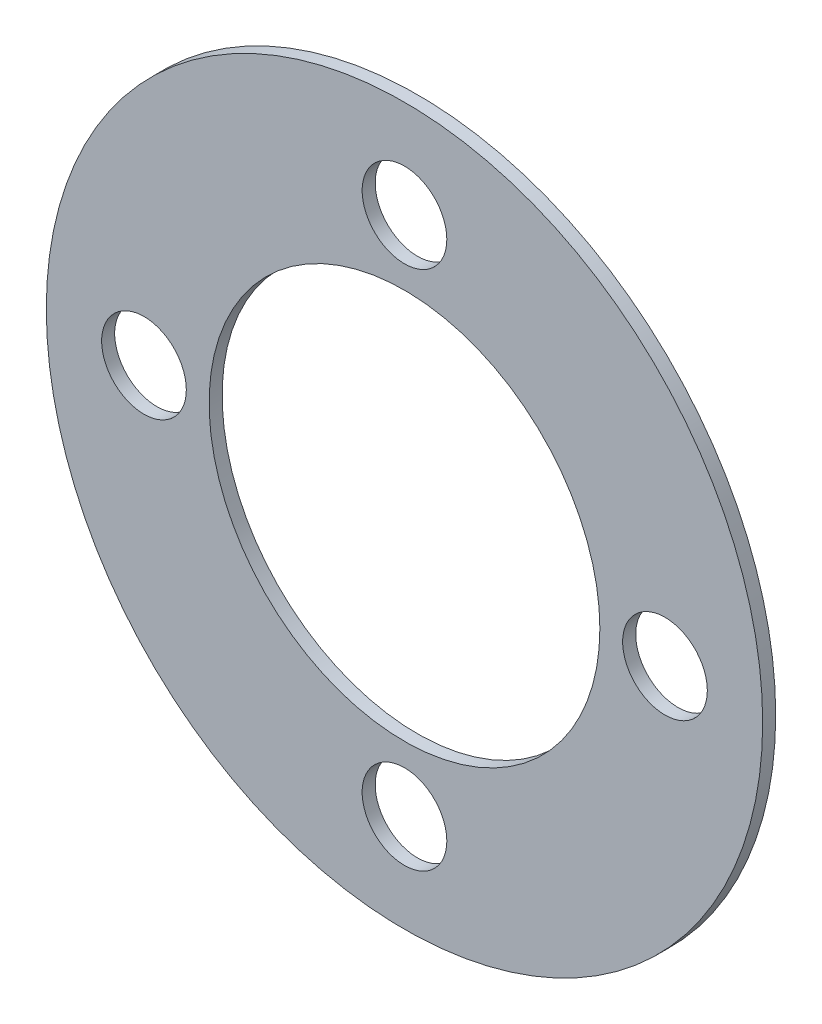
SolidWorks part; units mm, degrees
ref_plane "Front Plane" through (0, 0, 0) normal (0, 0, 1) x (1, 0, 0)
ref_plane "Top Plane" through (0, 0, 0) normal (0, 1, 0) x (1, 0, 0)
ref_plane "Right Plane" through (0, 0, 0) normal (1, 0, 0) x (0, 0, -1)
other "Configuration Table"
sketch "Sketch1" plane through (0, 0, 0) normal (0, 0, 1) x (1, 0, 0)
  line L0 (0, 0) -> (0, 33.134) construction
  circle A0 centre (0, 0) radius 27.5
  circle A1 centre (0, 0) radius 15
  circle A2 centre (0, 20) radius 3.25
  circle A3 centre (20, 0) radius 3.25
  circle A4 centre (0, -20) radius 3.25
  circle A5 centre (-20, 0) radius 3.25
  point P16 (0, 0)
  dimension "D1" = 55
  dimension "D2" = 30
  dimension "D4" = 6.5
  dimension "D3" = 20
  dimension "D5" = 4
extrude "Boss-Extrude1" add sketch "Sketch1" along normal blind 1
